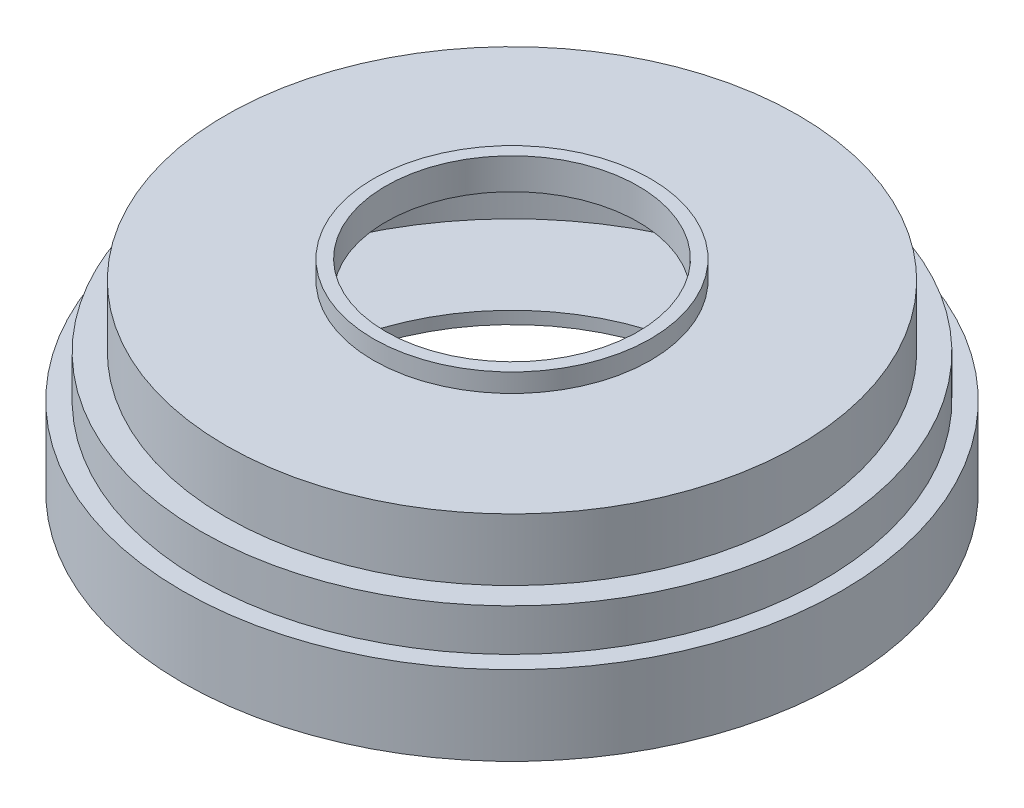
from build123d import *


with BuildPart() as part:
    # Sketch1 → Revolve1 (revolve)
    with BuildSketch(Plane.XY, mode=Mode.PRIVATE) as revolve1_sk:
        Polygon((43, 136), (43, 141), (53, 141), (53, 153.772755302), (50, 153.772755302), (50, 160.531936258), (46, 160.531936258), (46, 170.5), (22.284123589, 170.5), (22.284123589, 173.5), (20.284123589, 173.5), (20.284123589, 168.5), (44, 168.5), (44, 158.531936258), (48, 158.531936258), (48, 151.772755302), (51, 151.772755302), (51, 143), (41, 143), (33, 143), (33, 141), (41, 141), (41, 136), align=None)
    revolve(revolve1_sk.sketch.rotate(Axis((0, 0, 0), (0, -1, 0)), 90), axis=Axis((0, 0, 0), (0, -1, 0)))


solid = part.part
